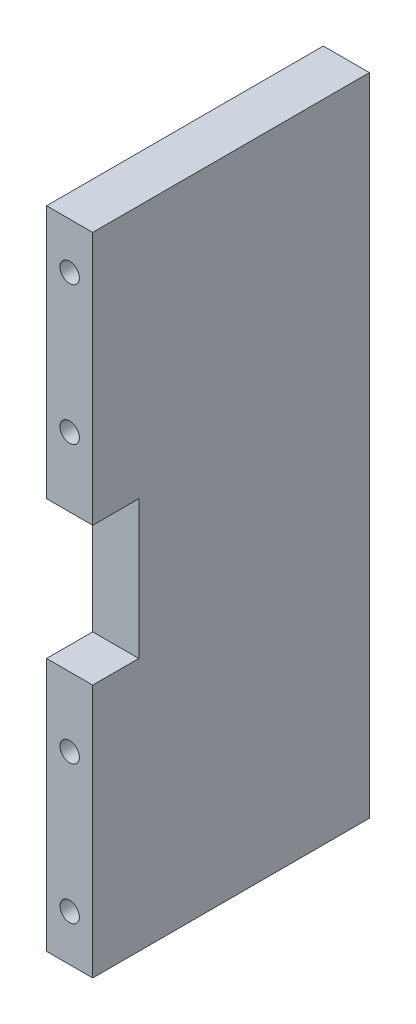
SolidWorks part; units mm, degrees
material "6061 Alloy"
ref_plane "Front Plane" through (0, 0, 0) normal (0, 0, 1) x (1, 0, 0)
ref_plane "Top Plane" through (0, 0, 0) normal (0, 1, 0) x (1, 0, 0)
ref_plane "Right Plane" through (0, 0, 0) normal (1, 0, 0) x (0, 0, -1)
sketch "Sketch 1" plane through (0, 0, 0) normal (1, 0, 0) x (0, 0, -1)
  line L1 (-30, -70) -> (30, -70)
  line L2 (-30, -70) -> (-30, 70)
  line L3 (-30, 70) -> (30, 70)
  line L4 (30, -70) -> (30, 70)
  line L5 (-30, -70) -> (30, 70) construction
  line L6 (-30, 70) -> (30, -70) construction
  point P0 (0, 0)
  dimension "D1" = 60
  dimension "D2" = 140
extrude "Boss-Extrude 1" add sketch "Sketch 1" along normal blind 10
sketch "Sketch 4" plane through (0, 0, 0) normal (-1, 0, 0) x (0, 0, 1)
  line L0 (30, 70) -> (30, -70) construction
  line L1 (30, -15) -> (20, -15)
  line L2 (30, -15) -> (30, 15)
  line L3 (30, 15) -> (20, 15)
  line L4 (20, -15) -> (20, 15)
  line L5 (30, -70) -> (-30, -70) construction
  dimension "D1" = 30
  dimension "D2" = 55
  dimension "D3" = 10
extrude "Cut-Extrude 1" cut sketch "Sketch 4" against normal through all
hole_wizard "M5 Tapped Hole 2" positions "Sketch 6" profile "Sketch 5" tap size "M5" standard "GB"
sketch "Sketch 6" plane through (0, 0, -30) normal (0, 0, -1) x (-1, 0, 0)
  line L0 (-10, -70) -> (-10, 70) construction
  line L1 (0, -70) -> (0, 70) construction
  point P0 (-5, 60)
  point P3 (0, 0)
  dimension "D1" = 5
  dimension "D2" = 60
sketch "Sketch 5" plane through (5, 60, -30) normal (1, 0, 0) x (0, 1, 0)
  line L0 (0, 0) -> (0, 13.6618)
  line L1 (0, 13.6618) -> (2.1, 12.4)
  line L2 (2.1, 12.4) -> (2.1, 0)
  line L5 (2.1, 0) -> (0, 0)
  line L10 (0, 13.6618) -> (-2.1, 12.4) construction
  line L11 (0, -6.35) -> (0, 107.95) construction
  dimension "螺孔鑽直徑" = 4.2
  dimension "螺孔鑽深度" = 12.4
  dimension "導頭角度" = 118
cosmetic thread "Cosmetic Thread 2" parameters "D1"=10, "D2"=5
pattern_linear "Linear Pattern 2" count 3 spacing 60 along (0, -1, 0) of "M5 Tapped Hole 2"
hole_wizard "M5 Tapped Hole 3" positions "Sketch 8" profile "Sketch 7" tap size "M5" standard "GB"
sketch "Sketch 8" plane through (0, 0, 30) normal (0, 0, 1) x (1, 0, 0)
  line L0 (10, -70) -> (0, -70) construction
  line L1 (10, 70) -> (0, 70) construction
  line L2 (10, -15) -> (10, -70) construction
  point P0 (5, -60)
  point P1 (5, -30)
  point P3 (5, 30)
  point P5 (5, 60)
  dimension "D1" = 10
  dimension "D2" = 30
  dimension "D3" = 10
  dimension "D4" = 30
  dimension "D5" = 5
sketch "Sketch 7" plane through (5, -60, 30) normal (1, 0, 0) x (0, -1, 0)
  line L0 (0, 0) -> (0, 13.6618)
  line L1 (0, 13.6618) -> (2.1, 12.4)
  line L2 (2.1, 12.4) -> (2.1, 0)
  line L5 (2.1, 0) -> (0, 0)
  line L10 (0, 13.6618) -> (-2.1, 12.4) construction
  line L11 (0, -6.35) -> (0, 107.95) construction
  dimension "螺孔鑽直徑" = 4.2
  dimension "螺孔鑽深度" = 12.4
  dimension "導頭角度" = 118
cosmetic thread "Cosmetic Thread 3" parameters "D1"=10, "D2"=5
cosmetic thread "Cosmetic Thread 4" parameters "D1"=10, "D2"=5
cosmetic thread "Cosmetic Thread 5" parameters "D1"=10, "D2"=5
cosmetic thread "Cosmetic Thread 6" parameters "D1"=10, "D2"=5
